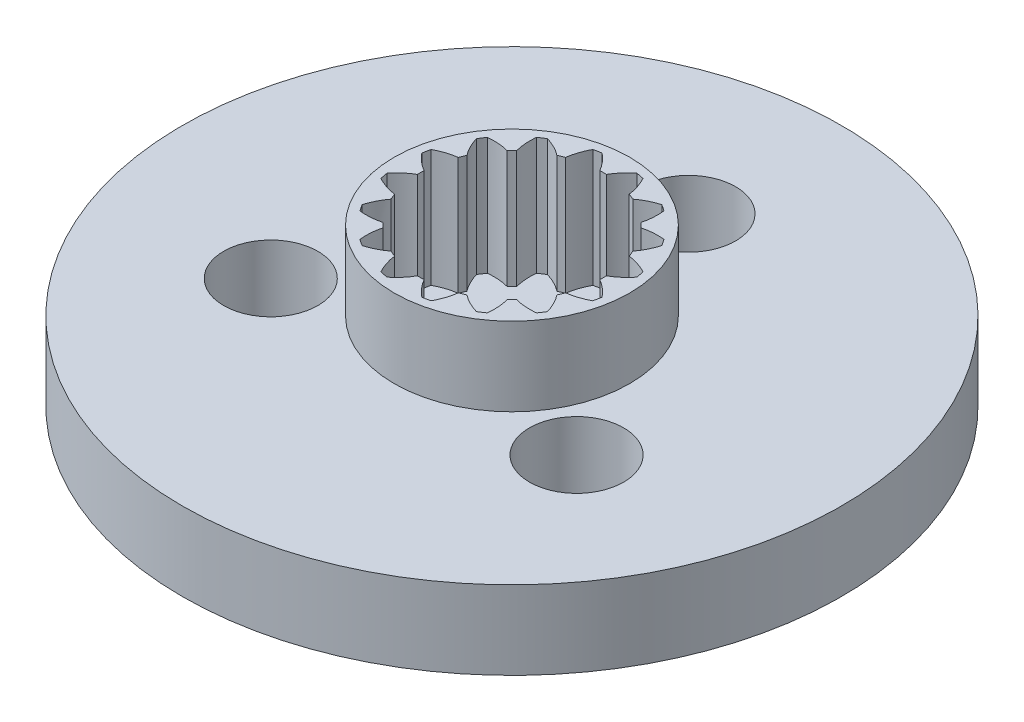
from build123d import *

# Parameters (mm, degrees)
SKETCH1_R                = 42
SKETCH1_R_2              = 6
SKETCH1_R_3              = 14
BOSS_EXTRUDE1_DEPTH      = 5
BOSS_EXTRUDE4_DEPTH      = 10
BOSS_EXTRUDE4_DEPTH_BACK = 10
SKETCH_2_5_R             = 15
SKETCH_2_5_R_2           = 13.875
BOSS_EXTRUDE5_START      = -5
BOSS_EXTRUDE5_DEPTH      = 15
CIRPATTERN3_COUNT        = 16
SKETCH3_R                = 15.986254567
BOSS_EXTRUDE6_DEPTH      = 3


with BuildPart() as part:
    # Sketch1 → Boss-Extrude1 (new, symmetric)
    with BuildSketch(Plane(origin=(0, 0, 0), x_dir=(1, 0, 0), z_dir=(0, 1, 0))):
        with Locations(Location((0, 0, 0), (0, 0, 270))):
            Circle(SKETCH1_R)
        with Locations(Location((0, 22.5, 0), (0, 0, 270))):
            Circle(SKETCH1_R_2, mode=Mode.SUBTRACT)
        with Locations(Location((19.485571585, -11.25, 0), (0, 0, 270))):
            Circle(SKETCH1_R_2, mode=Mode.SUBTRACT)
        with Locations(Location((-19.485571585, -11.25, 0), (0, 0, 270))):
            Circle(SKETCH1_R_2, mode=Mode.SUBTRACT)
        with Locations(Location((0, 0, 0), (0, 0, 270))):
            Circle(SKETCH1_R_3, mode=Mode.SUBTRACT)
    extrude(amount=BOSS_EXTRUDE1_DEPTH, both=True)

    # Sketch 2_5 → Boss-Extrude4 (add, two sides: drawn at the far end of the back side and taken through both)
    with BuildSketch(Plane(origin=(0, 5, 0), x_dir=(1, 0, 0), z_dir=(0, 1, 0)).offset(-BOSS_EXTRUDE4_DEPTH_BACK)):
        with Locations(Location((0, 0, 0), (0, 0, 270))):
            Circle(SKETCH_2_5_R)
        with Locations(Location((0, 0, 0), (0, 0, 270))):
            Circle(SKETCH_2_5_R_2, mode=Mode.SUBTRACT)
    extrude(amount=BOSS_EXTRUDE4_DEPTH + BOSS_EXTRUDE4_DEPTH_BACK)

    # Sketch 2_5 2 → Boss-Extrude5 (add)
    with BuildSketch(Plane(origin=(0, 5, 0), x_dir=(1, 0, 0), z_dir=(0, 1, 0)).offset(BOSS_EXTRUDE5_START)):
        with BuildLine():
            ThreePointArc((13.696966795, -2.215564403), (13.830420082, -1.111352942), (13.875, 0))
            ThreePointArc((13.875, 0), (13.830420082, 1.111352942), (13.696966795, 2.215564403))
            add(Edge.make_bspline(
                [(11.617209173, 0.425530281), (11.701464362, 0.47170702), (12.013646007, 0.652925794), (12.541420383, 1.022746254), (13.055086051, 1.487082264), (13.456629936, 1.92565845), (13.666997571, 2.178969311), (13.696966795, 2.215564403)],
                knots=[0.023147466, 0.023147466, 0.023147466, 0.023147466, 0.023147466, 0.029959916, 0.048733667, 0.068727063, 0.072081018, 0.072081018, 0.072081018, 0.072081018, 0.072081018], degree=4))
            ThreePointArc((11.617209173, 0.425530281), (11.62305213, 0.212800797), (11.625, 0))
            ThreePointArc((11.625, 0), (11.62305213, -0.212800797), (11.617209173, -0.425530281))
            add(Edge.make_bspline(
                [(11.617209173, -0.425530281), (11.701464362, -0.47170702), (12.013646007, -0.652925794), (12.541420383, -1.022746254), (13.055086051, -1.487082264), (13.456629936, -1.92565845), (13.666997571, -2.178969311), (13.696966795, -2.215564403)],
                knots=[0.023147466, 0.023147466, 0.023147466, 0.023147466, 0.023147466, 0.029959916, 0.048733667, 0.068727063, 0.072081018, 0.072081018, 0.072081018, 0.072081018, 0.072081018], degree=4))
        make_face()
    boss_extrude5 = extrude(amount=BOSS_EXTRUDE5_DEPTH)

    # CirPattern3: Boss-Extrude5 ×16 about axis
    cirpattern3_axis = Axis((0, 0, 0), (0, 1, 0))
    for i in range(1, CIRPATTERN3_COUNT):
        add(boss_extrude5.rotate(cirpattern3_axis, i * 360 / CIRPATTERN3_COUNT))

    # Sketch3 → Boss-Extrude6 (add)
    with BuildSketch(Plane.XZ):
        Circle(SKETCH3_R)
    extrude(amount=BOSS_EXTRUDE6_DEPTH)


solid = part.part
